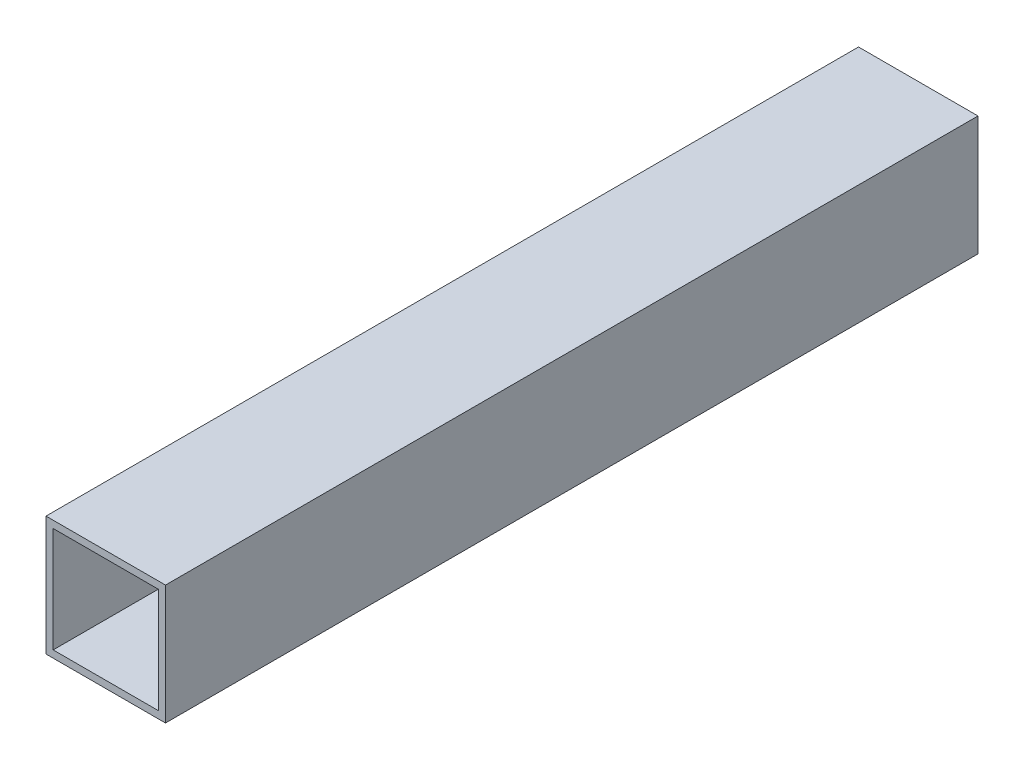
from build123d import *

# Parameters (mm, degrees)
SKETCH_1_W      = 50
SKETCH_1_H      = 50
SKETCH_1_W_2    = 44
SKETCH_1_H_2    = 44
EXTRUDE_2_DEPTH = 340


with BuildPart() as part:
    # 草图1 → 凸台-拉伸2 (new body)
    with BuildSketch(Plane.XY):
        with Locations((25, 25)):
            Rectangle(SKETCH_1_W, SKETCH_1_H)
        with Locations((25, 25)):
            Rectangle(SKETCH_1_W_2, SKETCH_1_H_2, mode=Mode.SUBTRACT)
    extrude(amount=EXTRUDE_2_DEPTH)


solid = part.part
